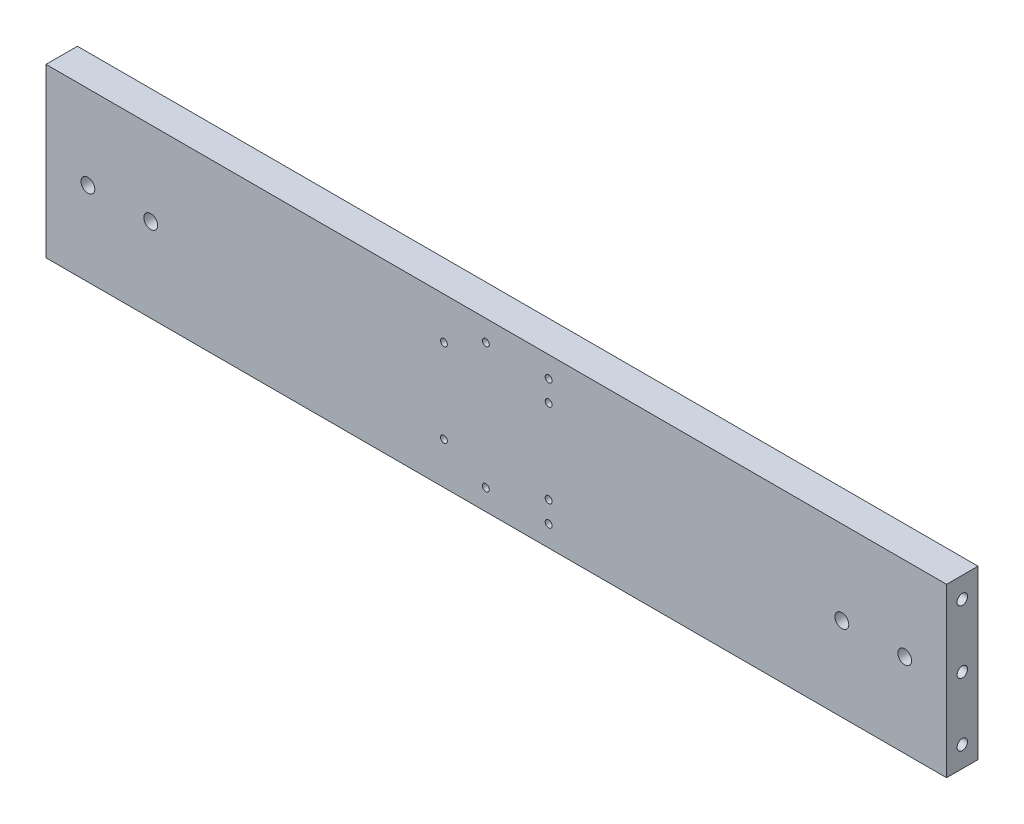
SolidWorks part; units mm, degrees
ref_plane "前视基准面" through (0, 0, 0) normal (0, 0, 1) x (1, 0, 0)
ref_plane "上视基准面" through (0, 0, 0) normal (0, 1, 0) x (1, 0, 0)
ref_plane "右视基准面" through (0, 0, 0) normal (1, 0, 0) x (0, 0, -1)
sketch "草图1" plane through (0, 0, 0) normal (0, 0, 1) x (1, 0, 0)
  line L1 (215, 40) -> (-215, 40)
  line L2 (215, 40) -> (215, -40)
  line L3 (215, -40) -> (-215, -40)
  line L4 (-215, 40) -> (-215, -40)
  line L5 (215, 40) -> (-215, -40) construction
  line L6 (215, -40) -> (-215, 40) construction
  point P0 (0, 0)
  dimension "D1" = 430
  dimension "D2" = 80
extrude "凸台-拉伸1" add sketch "草图1" along normal blind 15
ref_plane "基准面1" through (0, 0, 0) normal (0, 1, 0) x (1, 0, 0)
hole_wizard "M4 螺纹孔6" positions "草图23" profile "草图24" tap size "M4" standard "ISO" end condition through all
sketch "草图23" plane through (0, 0, 0) normal (0, 0, 1) x (1, 0, 0)
  line L0 (0, 40) -> (0, -40) construction
  line L1 (215, 40) -> (-215, 40) construction
  line L2 (-215, -40) -> (215, -40) construction
  line L3 (0, 0) -> (49.8421, 0) construction
  point P0 (25, -20)
  point P2 (-25, -20)
  point P4 (-25, 20)
  point P6 (25, 20)
  dimension "D1" = 50
  dimension "D2" = 40
sketch "草图24" plane through (25, -20, 0) normal (1, 0, 0) x (0, 1, 0)
  line L0 (0, 0) -> (0, 15)
  line L1 (0, 15) -> (1.65, 15)
  line L2 (1.65, 15) -> (1.65, 0)
  line L5 (1.65, 0) -> (0, 0)
  line L11 (0, -6.35) -> (0, 107.95) construction
  dimension "通孔螺纹孔钻头直径" = 3.3
  dimension "通孔螺纹孔钻头深度" = 15
cosmetic thread "孔螺蚊线21" parameters "D2"=4
cosmetic thread "孔螺蚊线22" parameters "D2"=4
cosmetic thread "孔螺蚊线23" parameters "D2"=4
cosmetic thread "孔螺蚊线24" parameters "D2"=4
hole_wizard "M4 螺纹孔7" positions "草图27" profile "草图29" tap size "M4" standard "ISO" end condition through all
sketch "草图27" plane through (0, 0, 0) normal (0, 0, -1) x (-1, 0, 0)
  circle A0 centre (-25, 30) radius 4 construction
  circle A1 centre (-25, -30) radius 4 construction
  circle A2 centre (5, -30) radius 4 construction
  circle A3 centre (5, 30) radius 4 construction
  point P0 (5, 30)
  point P2 (5, -30)
  point P4 (-25, 30)
  point P6 (-25, -30)
sketch "草图29" plane through (-5, 30, 0) normal (1, 0, 0) x (0, 1, 0)
  line L0 (0, 0) -> (0, 15)
  line L1 (0, 15) -> (1.65, 15)
  line L2 (1.65, 15) -> (1.65, 0)
  line L5 (1.65, 0) -> (0, 0)
  line L11 (0, -6.35) -> (0, 107.95) construction
  dimension "通孔螺纹孔钻头直径" = 3.3
  dimension "通孔螺纹孔钻头深度" = 15
cosmetic thread "孔螺蚊线31" parameters "D2"=4
cosmetic thread "孔螺蚊线32" parameters "D2"=4
cosmetic thread "孔螺蚊线33" parameters "D2"=4
cosmetic thread "孔螺蚊线34" parameters "D2"=4
hole_wizard "M4 螺纹孔8" positions "草图30" profile "草图31" tap size "M4" standard "ISO"
sketch "草图30" plane through (0, 0, 0) normal (0, 0, -1) x (-1, 0, 0)
  line L0 (0, 0) -> (0, 40) construction
  line L1 (-190, 40) -> (190, 40) construction
  line L3 (0, 0) -> (41.993, 0) construction
  point P0 (-42, 22.5)
  point P2 (-42, -22.5)
  point P4 (42, 22.5)
  point P6 (42, -22.5)
  dimension "D1" = 84
  dimension "D2" = 45
sketch "草图31" plane through (42, 22.5, 0) normal (1, 0, 0) x (0, 1, 0)
  line L0 (0, 0) -> (0, 15)
  line L1 (0, 15) -> (1.65, 15)
  line L2 (1.65, 15) -> (1.65, 0)
  line L5 (1.65, 0) -> (0, 0)
  line L11 (0, -6.35) -> (0, 107.95) construction
  dimension "通孔螺纹孔钻头直径" = 3.3
  dimension "通孔螺纹孔钻头深度" = 15
cosmetic thread "孔螺蚊线35" [suppressed] parameters "D2"=4
cosmetic thread "孔螺蚊线36" [suppressed] parameters "D2"=4
cosmetic thread "孔螺蚊线37" [suppressed] parameters "D2"=4
cosmetic thread "孔螺蚊线38" [suppressed] parameters "D2"=4
hole_wizard "M4 六角凹头螺钉的柱形沉头孔5" positions "草图32" profile "草图33" counterbore size "M6" standard "ISO" end condition through all
sketch "草图32" plane through (0, 0, 0) normal (0, 0, -1) x (-1, 0, 0)
  circle A0 centre (195, 0) radius 2.5 construction
  circle A1 centre (165, 0) radius 2.5 construction
  circle A2 centre (-165, 0) radius 2.5 construction
  circle A3 centre (-195, 0) radius 2.5 construction
  point P0 (-195, 0)
  point P2 (-165, 0)
  point P4 (165, 0)
  point P6 (195, 0)
sketch "草图33" plane through (195, 0, 0) normal (1, 0, 0) x (0, 1, 0)
  line L0 (0, 0) -> (0, 15)
  line L1 (0, 15) -> (3.3, 15)
  line L3 (3.3, 15) -> (3.3, 6.4)
  line L4 (3.3, 6.4) -> (5.5, 6.4)
  line L5 (5.5, 6.4) -> (5.5, 0)
  line L7 (5.5, 0) -> (0, 0)
  line L11 (0, -6.35) -> (0, 107.95) construction
  dimension "通孔孔直径" = 6.6
  dimension "通孔孔深度" = 15
  dimension "柱形沉头孔直径" = 11
  dimension "柱形沉头孔深度" = 6.4
hole_wizard "M6 螺纹孔1" positions "草图34" profile "草图35" tap size "M6" standard "ISO"
sketch "草图34" plane through (215, 0, 0) normal (1, 0, 0) x (0, 0, -1)
  line L0 (-7.5, 40) -> (-7.5, -40) construction
  line L1 (-15, 40) -> (0, 40) construction
  line L2 (-15, -40) -> (0, -40) construction
  line L4 (0, 0) -> (-15, 0) construction
  line L5 (0, -40) -> (0, 40) construction
  line L6 (-15, -40) -> (-15, 40) construction
  point P0 (-7.5, 30)
  point P2 (-7.5, 0)
  point P4 (-7.5, -30)
  dimension "D1" = 60
sketch "草图35" plane through (215, 30, 7.5) normal (0, 1, 0) x (0, 0, -1)
  line L0 (0, 0) -> (0, 21.5022)
  line L1 (0, 21.5022) -> (2.5, 20)
  line L2 (2.5, 20) -> (2.5, 0)
  line L5 (2.5, 0) -> (0, 0)
  line L10 (0, 21.5022) -> (-2.5, 20) construction
  line L11 (0, -6.35) -> (0, 107.95) construction
  dimension "螺纹孔钻头直径" = 5
  dimension "螺纹孔钻头深度" = 20
  dimension "导头角度" = 118
cosmetic thread "孔螺蚊线39" parameters "D1"=19, "D2"=6
cosmetic thread "孔螺蚊线40" parameters "D1"=19, "D2"=6
cosmetic thread "孔螺蚊线41" parameters "D1"=19, "D2"=6
mirror "镜向1" about plane through (0, 0, 0) normal (1, 0, 0) of "M6 螺纹孔1"
